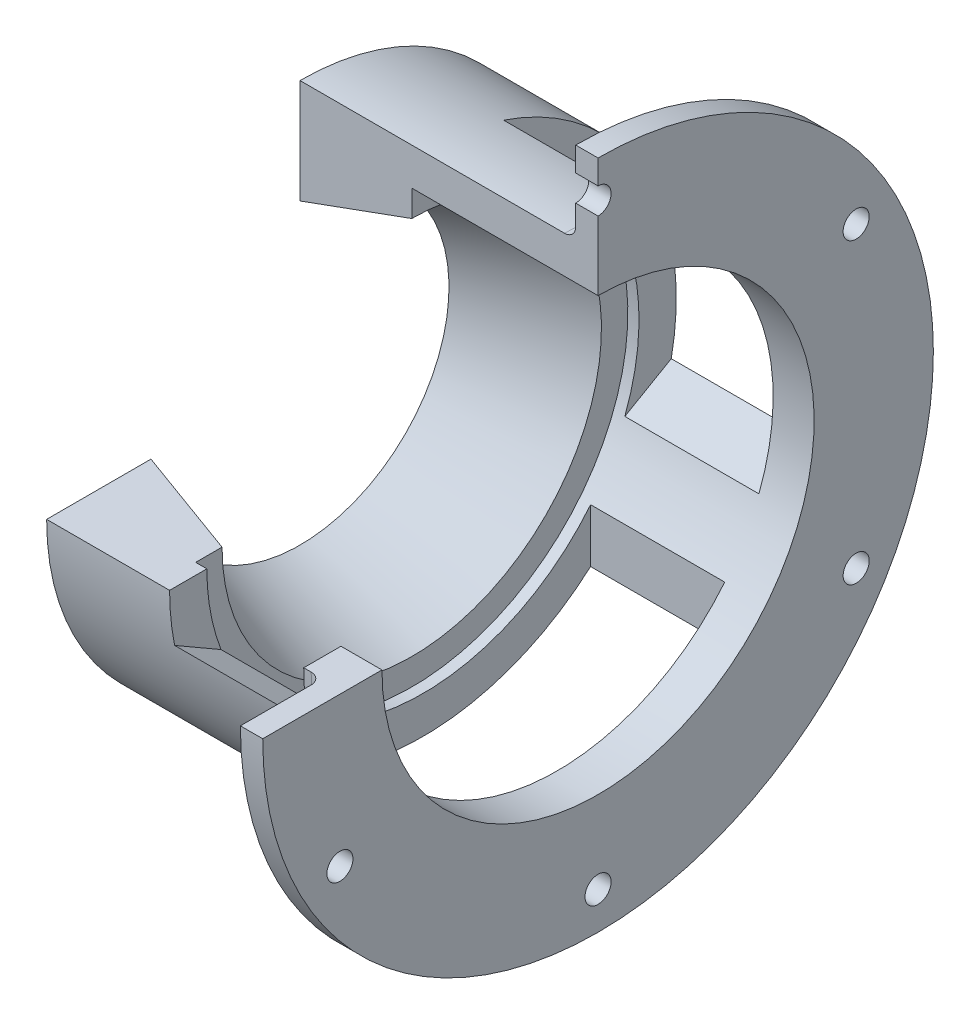
SolidWorks part; units mm, degrees
ref_plane "Front Plane" through (0, 0, 0) normal (0, 0, 1) x (1, 0, 0)
ref_plane "Top Plane" through (0, 0, 0) normal (0, 1, 0) x (1, 0, 0)
ref_plane "Right Plane" through (0, 0, 0) normal (1, 0, 0) x (0, 0, -1)
sketch "Sketch1" plane through (0, 0, 0) normal (0, 0, 1) x (1, 0, 0)
  line L0 (0, 0) -> (50.27, 0) construction
  line L1 (0, 40) -> (0, 68)
  line L2 (0, 68) -> (74, 68)
  line L3 (74, 68) -> (74, 90)
  line L4 (74, 90) -> (80, 90)
  line L5 (80, 90) -> (80, 58)
  line L6 (80, 58) -> (30, 58)
  line L7 (30, 50.9191) -> (0, 40)
  line L8 (30, 50.9191) -> (30, 58)
  dimension "D1" = 90
  dimension "D2" = 22
  dimension "D3" = 10
  dimension "D4" = 80
  dimension "D5" = 6
  dimension "D6" = 20
  dimension "D7" = 40
  dimension "D8" = 30
revolve "Revolve1" add sketch "Sketch1" angle 360 about L0
sketch "Sketch2" plane through (80, 0, 0) normal (1, 0, 0) x (0, 0, -1)
  circle A0 centre (0, 0) radius 80 construction
  circle A1 centre (0, 80) radius 3.5
  circle A2 centre (69.282, 40) radius 3.5
  circle A3 centre (69.282, -40) radius 3.5
  circle A4 centre (0, -80) radius 3.5
  circle A5 centre (-69.282, -40) radius 3.5
  circle A6 centre (-69.282, 40) radius 3.5
  point P18 (0, 0)
  dimension "D1" = 160
  dimension "D2" = 7
  dimension "D3" = 6
extrude "Cut-Extrude1" cut sketch "Sketch2" against normal blind 10
fillet "Fillet1" radius 3 1 edges at (74, 0, 68)
sketch "Sketch3" plane through (0, 0, 0) normal (0, 1, 0) x (1, 0, 0)
  line L0 (74, 71) -> (74, -71) construction
  line L1 (33, 45) -> (69, 45)
  line L2 (33, 45) -> (33, -45)
  line L3 (33, -45) -> (69, -45)
  line L4 (69, 45) -> (69, -45)
  line L5 (33, 45) -> (69, -45) construction
  line L6 (33, -45) -> (69, 45) construction
  point P0 (51, 0)
  dimension "D1" = 36
  dimension "D2" = 90
  dimension "D3" = 5
  dimension "D4" = 0
extrude "Cut-Extrude2" cut sketch "Sketch3" against normal through all
pattern_circular "CirPattern1" count 3 over 360 about axis through (0, 0, 0) along (1, 0, 0) of "Cut-Extrude2"
sketch "Sketch4" plane through (0, 0, 0) normal (-1, 0, 0) x (0, 0, 1)
  line L1 (0, 0) -> (114.5788, 0)
  line L2 (0, 0) -> (0, 147.1584)
  line L3 (0, 147.1584) -> (114.5788, 147.1584)
  line L4 (114.5788, 0) -> (114.5788, 147.1584)
extrude "Cut-Extrude3" cut sketch "Sketch4" against normal through all
